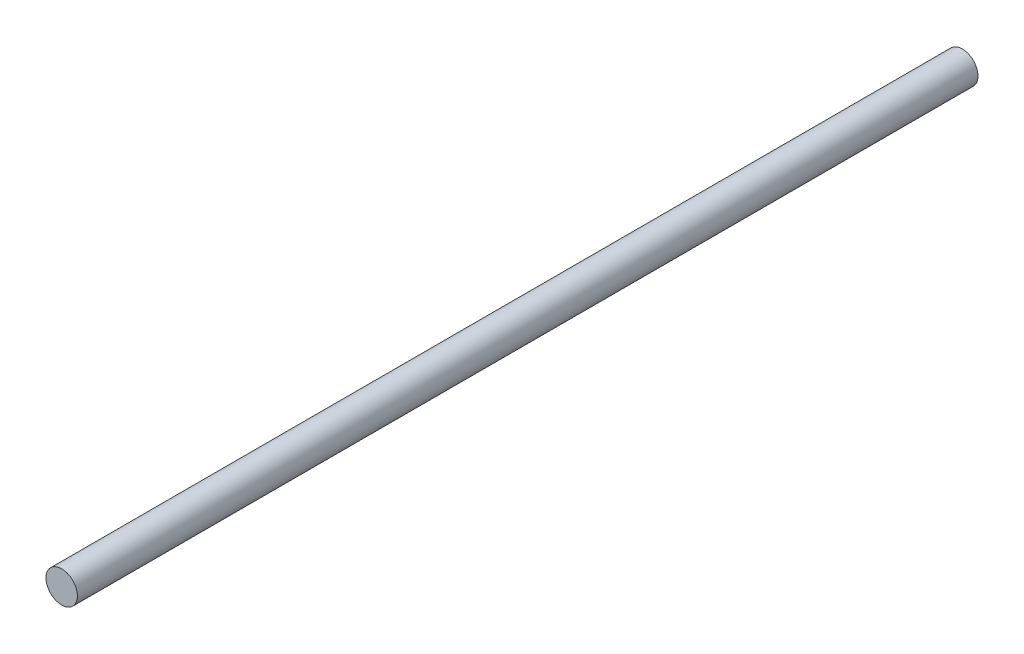
from build123d import *

# Parameters (mm, degrees)
SKETCH_1_R      = 7.5
EXTRUDE_1_DEPTH = 430


with BuildPart() as part:
    # 草图1 → 凸台-拉伸1 (new body)
    with BuildSketch(Plane.XY):
        Circle(SKETCH_1_R)
    extrude(amount=EXTRUDE_1_DEPTH)


solid = part.part
